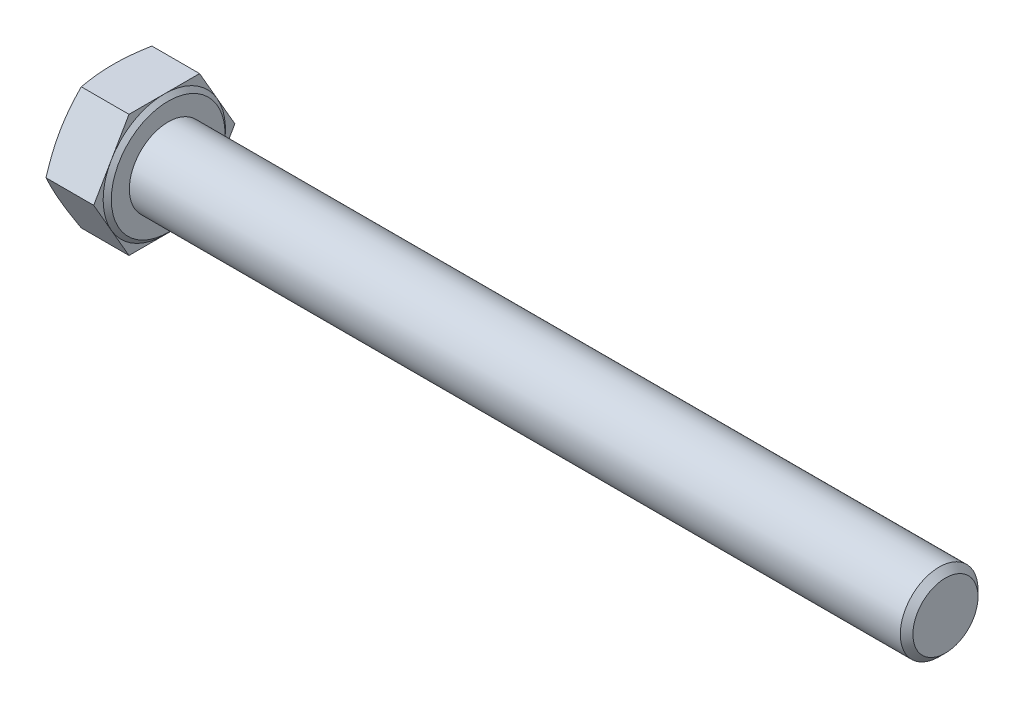
SolidWorks part; units mm, degrees
ref_plane "Front" through (0, 0, 0) normal (0, 0, 1) x (1, 0, 0)
ref_plane "Top" through (0, 0, 0) normal (0, 1, 0) x (1, 0, 0)
ref_plane "Right" through (0, 0, 0) normal (1, 0, 0) x (0, 0, -1)
sketch "Sketch-BaseHead" plane through (0, 0, 0) normal (1, 0, 0) x (0, 0, -1)
  line L1 (9.0817, 0) -> (4.5409, 7.865)
  line L2 (4.5409, 7.865) -> (-4.5409, 7.865)
  line L3 (-4.5409, 7.865) -> (-9.0817, 0)
  line L4 (-9.0817, 0) -> (-4.5409, -7.865)
  line L5 (-4.5409, -7.865) -> (4.5409, -7.865)
  line L6 (4.5409, -7.865) -> (9.0817, 0)
  circle A0 centre (0, 0) radius 7.865 construction
extrude "BaseHead" add sketch "Sketch-BaseHead" along normal blind 6.58
sketch "Sketch4" plane through (-0.2646, 0, 5.9169) normal (0, 1, 0) x (0, 0, -1)
  line L0 (5.9169, 3.7369) -> (5.9169, -10.4477) construction
  line L2 (14.9986, -0.2646) -> (13.7819, -0.2646)
  line L4 (13.7819, -0.2646) -> (14.9986, -0.7075)
  line L6 (14.9986, -0.7075) -> (14.9986, -0.2646)
revolve "HeadChamfer" cut sketch "Sketch4" angle 360 about L0
sketch "Sketch1" plane through (0, 0, 0) normal (0, 0, 1) x (1, 0, 0)
  line L0 (6.58, 0) -> (7.08, 0)
  line L1 (7.08, 0) -> (7.08, -7.315)
  line L2 (7.08, -7.315) -> (6.58, -7.865)
  line L3 (6.58, -7.865) -> (6.58, 0) construction
  line L4 (0, 0) -> (7.5821, 0) construction
  line L5 (-4.0016, 0) -> (10.1831, 0) construction
  line L6 (6.58, -7.865) -> (0.4428, -7.865) construction
  line L7 (6.58, 0) -> (6.58, -7.865)
revolve "Revolve1" add sketch "Sketch1" angle 360 about axis through (-4.0016, 0, 0) along (1, 0, 0)
ref_plane "Plane2" through (81.08, 0, 0) normal (1, 0, 0) x (0, 0, -1)
sketch "Sketch3" plane through (7.08, 0, 0) normal (1, 0, 0) x (0, 0, -1)
  circle A0 centre (0, 0) radius 5
extrude "BaseBody" add sketch "Sketch3" along normal blind 100
cosmetic thread "ThreadCosmetic1" [suppressed] parameters "b"=26, "D2"=8.376
fillet "HeadFillet" [suppressed] radius 0.4
chamfer "Chamfer1" distance 0.812 angle 45 1 edges at (107.08, 0, -5)
sketch "Sketch5" plane through (0, 0, 0) normal (0, 0, 1) x (1, 0, 0)
  line L0 (105.456, 5.812) -> (106.268, 5.812)
  line L1 (106.268, 5.812) -> (106.268, 5)
  line L2 (106.268, 5) -> (105.862, 4.2968)
  line L3 (105.862, 4.2968) -> (105.456, 5)
  line L4 (105.456, 5) -> (105.456, 5.812)
  line L5 (106.268, -5) -> (106.268, 5) construction
  line L6 (106.268, 5) -> (7.08, 5) construction
revolve "Cut-Revolve10" [suppressed] cut sketch "Sketch5" angle 360
pattern_linear "LPattern10" [suppressed] count 27
equation "\"D1@Sketch1\" = \"s@Sketch-BaseHead\"/ 2"
equation "\"D2@Sketch4\" = \"s@Sketch-BaseHead\""
equation "\"D1@Chamfer1\" =  ( \"d@Sketch3\" - \"D2@ThreadCosmetic1\" ) / 2 "
equation "\"b@ThreadCosmetic1\" = \"l@BaseBody\" - \"lg@Plane2\""
equation "\"D1@Sketch5\" =  (\"d@Sketch3\" - \"D2@ThreadCosmetic1\" )  / 2 "
equation "\"pitch@LPattern10\" = 1.2 * \"D1@Sketch5\""
equation "\"D1@LPattern10\" = \"b@ThreadCosmetic1\" / \"pitch@LPattern10\""
